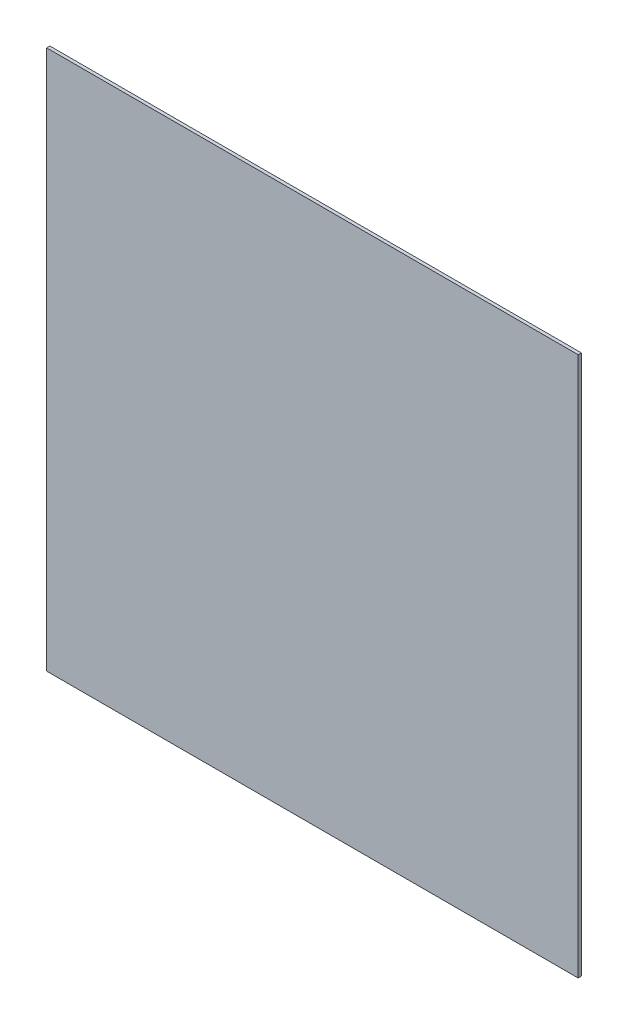
from build123d import *

# Parameters (mm, degrees)
SKETCH_1_W      = 829
SKETCH_1_H      = 842
EXTRUDE_1_DEPTH = 5


with BuildPart() as part:
    # 草图1 → 凸台-拉伸1 (new body)
    with BuildSketch(Plane.XY):
        Rectangle(SKETCH_1_W, SKETCH_1_H)
    extrude(amount=EXTRUDE_1_DEPTH)


solid = part.part
